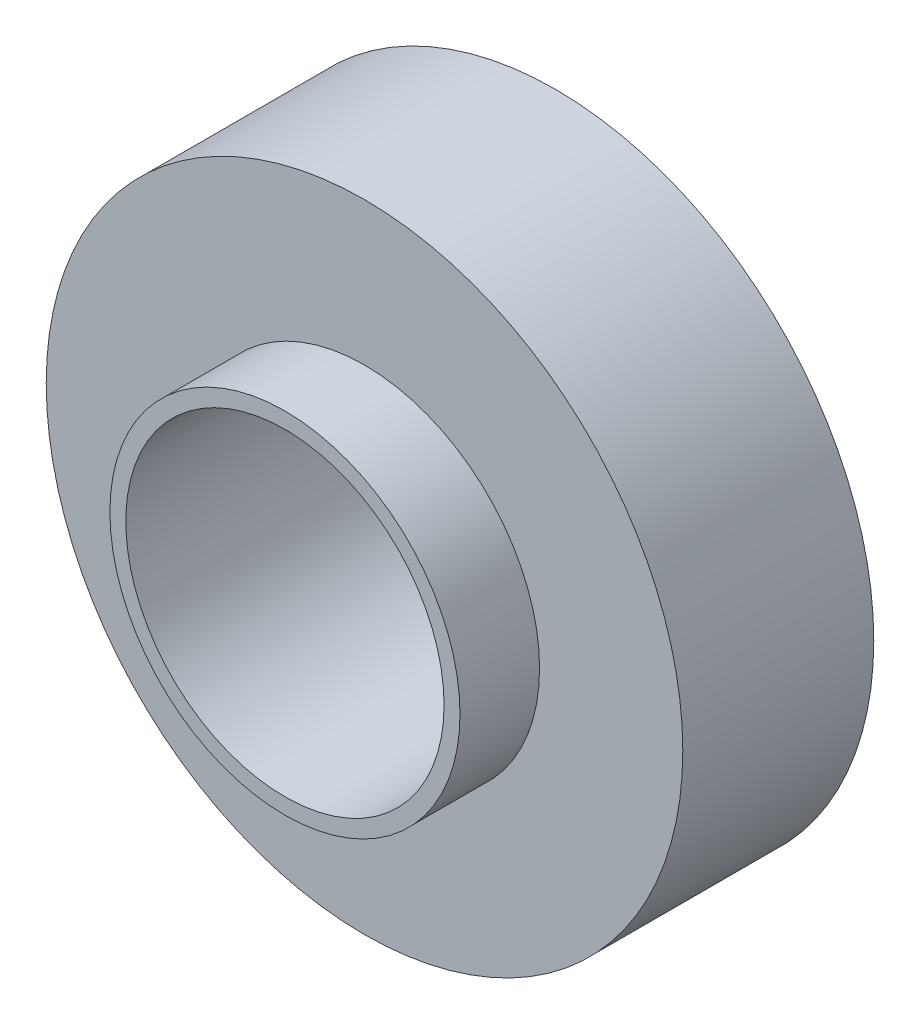
SolidWorks part; units mm, degrees
ref_plane "Front Plane" through (0, 0, 0) normal (0, 0, 1) x (1, 0, 0)
ref_plane "Top Plane" through (0, 0, 0) normal (0, 1, 0) x (1, 0, 0)
ref_plane "Right Plane" through (0, 0, 0) normal (1, 0, 0) x (0, 0, -1)
other "Configuration Table"
sketch "Sketch1" plane through (0, 0, 0) normal (0, 0, 1) x (1, 0, 0)
  circle A0 centre (0, 0) radius 10
  circle A1 centre (0, 0) radius 20
  dimension "D1" = 20
  dimension "D2" = 40
extrude "Boss-Extrude1" add sketch "Sketch1" along normal blind 12
sketch "Sketch2" plane through (0, 0, 12) normal (0, 0, 1) x (1, 0, 0)
  circle A1 centre (0, 0) radius 10 construction
  circle A2 centre (0, 0) radius 11
  circle A3 centre (0, 0) radius 11
  circle A4 centre (0, 0) radius 10
  dimension "D1" = 1
extrude "Boss-Extrude2" add sketch "Sketch2" along normal blind 5
